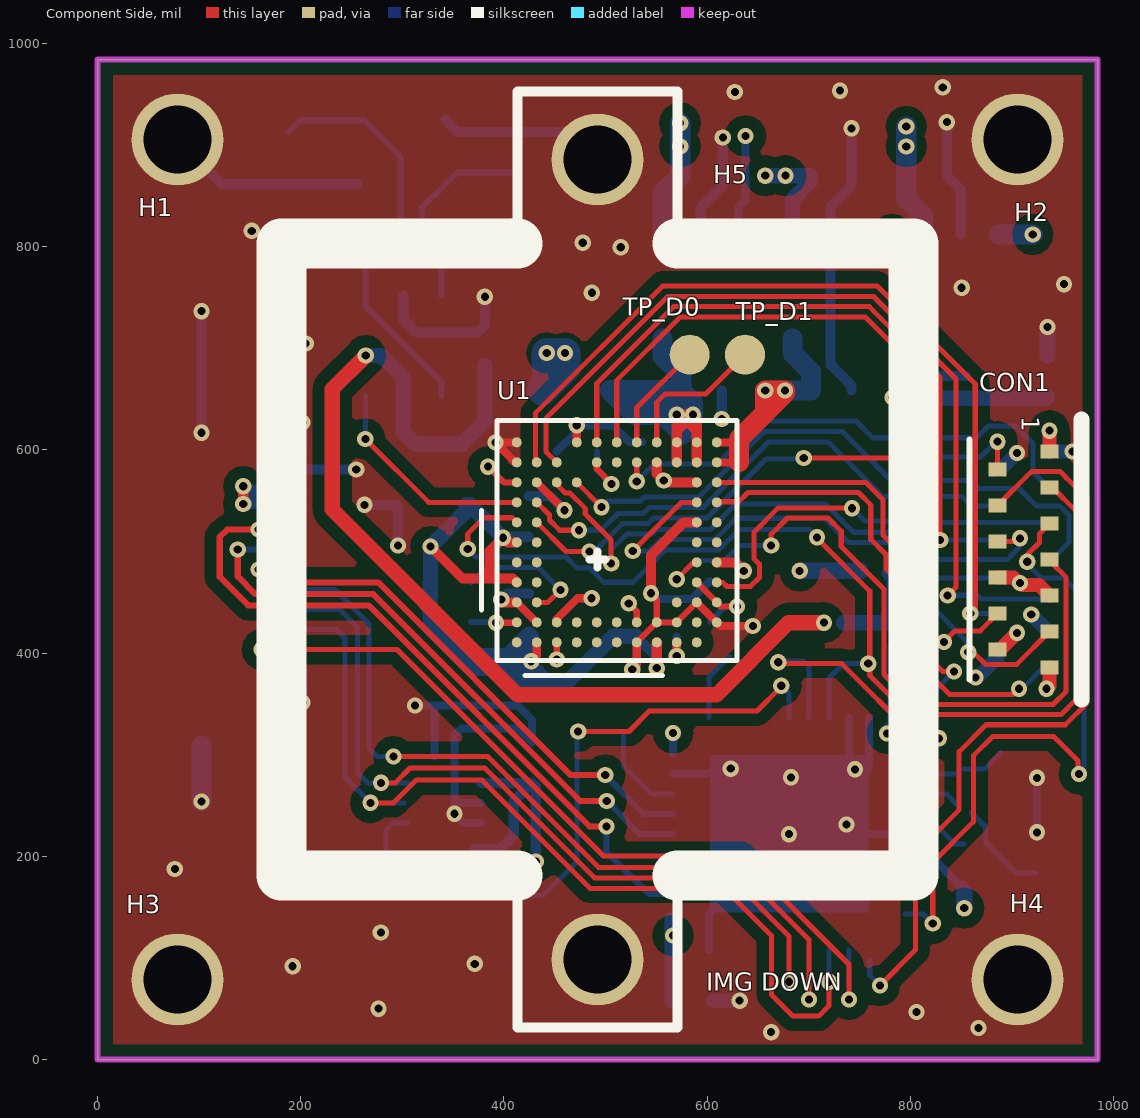
[diagram p0: Component Side view]
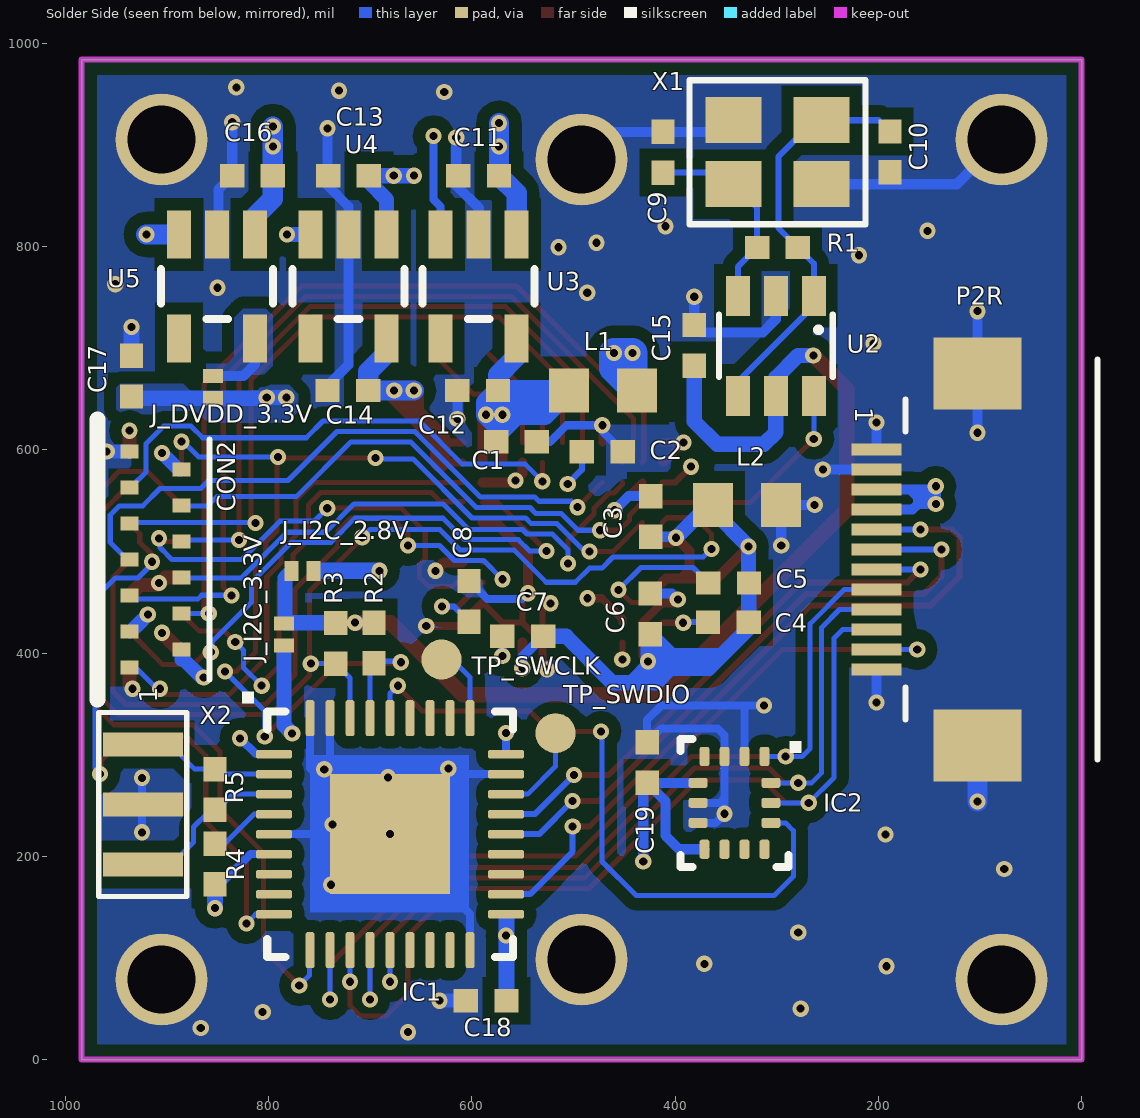
[diagram p1: Solder Side view, seen from below]
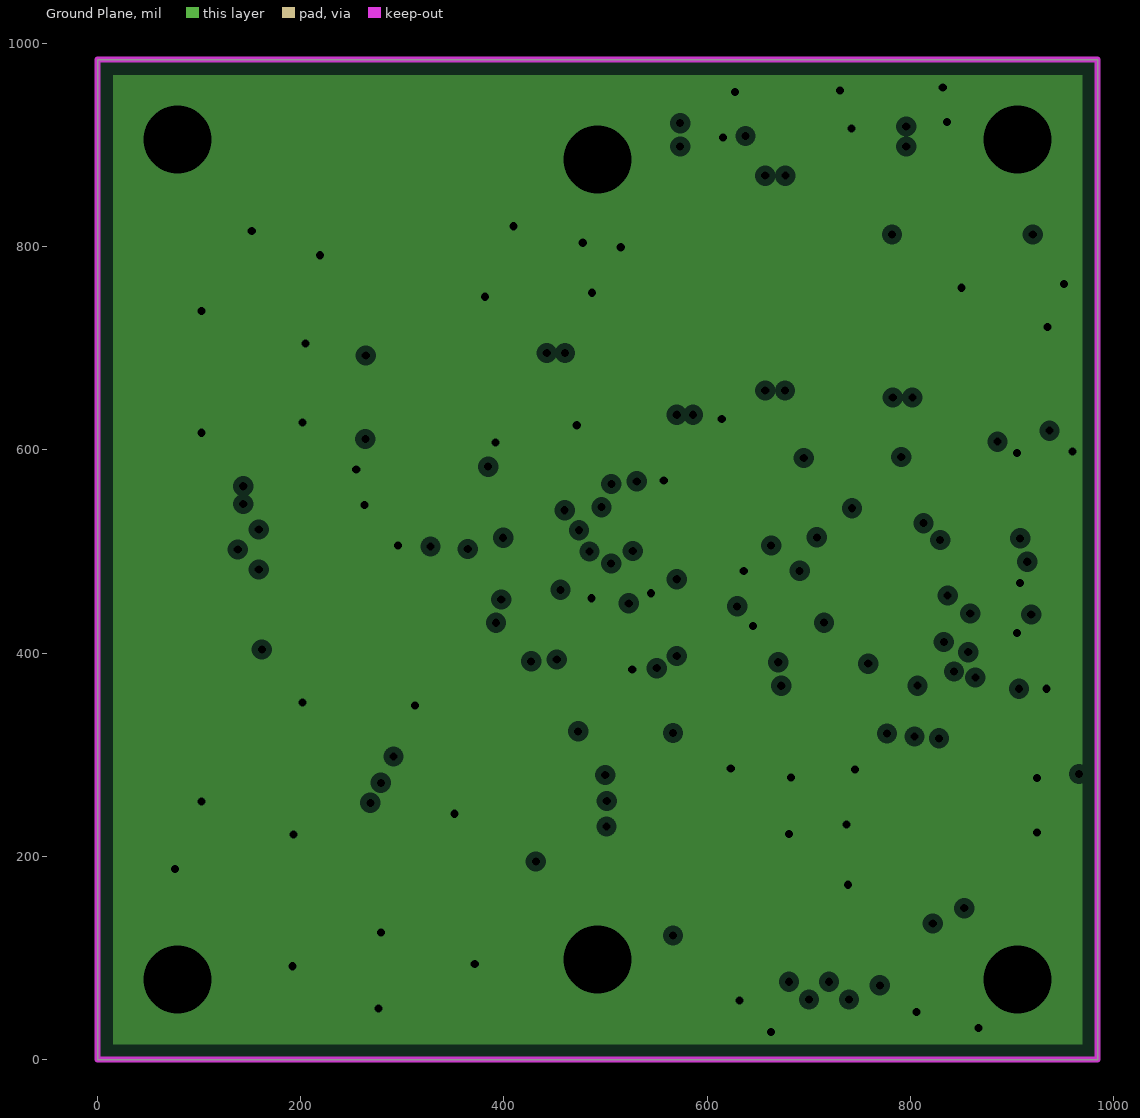
[diagram p2: Ground Plane, clearances drawn from the general rule]
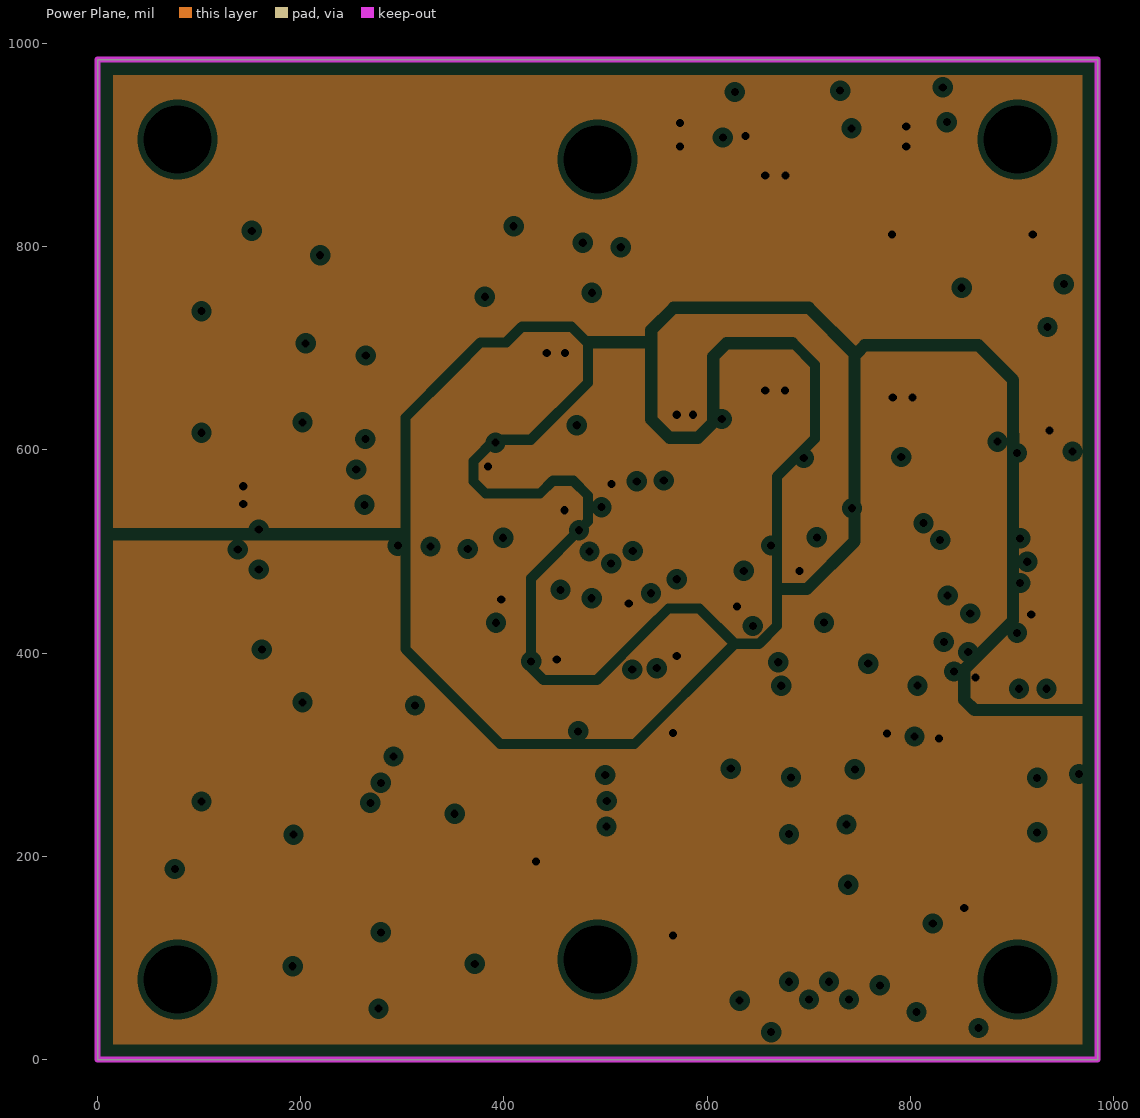
[diagram p3: Power Plane, clearances drawn from the general rule]
# Altium PCB MISC84416.PcbDoc
Units mil, origin at the board's own origin, x right, y up, seen from the top; angles counter-clockwise.
Board outline 984.25 x 984.25 mil, 4 copper layers (Component Side, Ground Plane, Power Plane, Solder Side), stack 33.234 mil thick; 50 components, 46 nets, 258 pads, 152 vias.

## Layer stack, top to bottom
Component Side: signal copper 1.4
Dielectric: core 12.6, FR-4, Dk 4.8
Ground Plane: plane copper 1.4169, net DGND
Dielectric: prepreg 5, Dk 4.2
Power Plane: plane copper 1.4169, net (Multiple Nets)
Dielectric: core 10, Dk 4.2
Solder Side: signal copper 1.4

## Board outline
0,0 984.25,0 984.25,984.25 0,984.25

## Design rules (kind name [scope] priority, off if disabled: settings)
AssemblyTestPointUsage [All] p1 off:
AssemblyTestpoint [All] p1 off: testpointundercomponent=TRUE minsize=40 maxsize=100 preferedsize=60 minholesize=0 maxholesize=40 preferedholesize=32 testpointgrid=1 usegrid=TRUE gridtolerance=0.01 allowsidetop=TRUE allowsidebottom=TRUE
Clearance Clearance_1 [InPolygon] p1: gap=12
Clearance [All] p2: gap=5
ComponentClearance [All] p1 off: gap=10 collisioncheckmode=3 verticalgap=10 showdistances=FALSE
DiffPairsRouting [All] p1 off: maxlimit=10 minlimit=10 mostfreqgap=10 maxuncoupledlength=500
FabricationTestPointUsage [All] p1 off: valid=0 allowmultiple=FALSE
FabricationTestpoint [All] p1 off: side=3 testpointundercomponent=TRUE minsize=40 maxsize=100 preferedsize=60 minholesize=0 maxholesize=40 preferedholesize=32 testpointgrid=1 allowsidetop=TRUE allowsidebottom=TRUE usegrid=TRUE gridtolerance=0.01
FanoutControl Fanout_BGA [IsBGA] p1 off: bgadir=Out bgaviamode=Centered fanoutstyle=Auto fanoutdirection=Alternating viagrid=1 // Fanout_BGA (Default Rule)
FanoutControl Fanout_LCC [IsLCC] p2 off: bgadir=Out bgaviamode=Centered fanoutstyle=Auto fanoutdirection=Alternating viagrid=1 // Fanout_LCC (Default Rule)
FanoutControl Fanout_SOIC [IsSOIC] p3 off: bgadir=Out bgaviamode=Centered fanoutstyle=Auto fanoutdirection=Alternating viagrid=1 // Fanout_SOIC (Default Rule)
FanoutControl Fanout_Small [(CompPinCount < 5)] p4 off: bgadir=Out bgaviamode=Centered fanoutstyle=Auto fanoutdirection=OutThenIn viagrid=1 // Fanout_Small (Default Rule)
FanoutControl Fanout_Default [All] p5 off: bgadir=Out bgaviamode=Centered fanoutstyle=Auto fanoutdirection=Alternating viagrid=1 // Fanout_Default (Default Rule)
Height [All] p1 off: minheight=0 maxheight=1000 prefheight=500
HoleSize [All] p1 off: absolutevalues=TRUE maxlimit=500 minlimit=1 maxpercent=80.000 minpercent=20.000
HoleToHoleClearance [All] p1 off: gap=0 allowstackedmicrovias=TRUE
LayerPairs [All] p1 off: enforce=TRUE
MinimumSolderMaskSliver [All] p1 off: minsoldermaskwidth=0
NetAntennae [All] p1 off: netantennaetolerance=0
PasteMaskExpansion [All] p1 off: expansion=0
PlaneClearance [All] p1: clearance=6
PlaneConnect [All] p1: planeconnectstyle=Direct reliefexpansion=20 reliefentries=4 reliefconductorwidth=10 reliefairgap=10
PolygonConnect [All] p1: connectstyle=Direct reliefconductorwidth=10 reliefentries=4 polygonreliefangle="90 Angle"
RoutingCorners [All] p1 off: cornerstyle=45-Degree minsetback=100 maxsetback=100
RoutingLayers [All] p1 off: top layer_v5=TRUE bottom layer_v5=TRUE
RoutingPriority [All] p1 off: routingpriority=0
RoutingTopology [All] p1 off: topology=Shortest
RoutingVias [All] p1: holewidth=8 width=16 viastyle="Through Hole" minholewidth=8 minwidth=16 maxholewidth=8 maxwidth=16
SilkToSilkClearance [All] p1 off: silktosilkclearance=0
SilkscreenOverComponentPads SilkToSolderMaskClearance [IsPad] p1 off: minsilkscreentomaskgap=0
SolderMaskExpansion [All] p1 off: expansion=4
Width [All] p1: maxlimit=200 minlimit=5 preferedwidth=5
2 further rules are at their usual default settings.

## Components (designator, comment, footprint, x,y, rotation, side; value= is the part's Value field where it differs from the comment)
C1 "1uF" RCL_C0402_TI 556.08,608 r180 bottom
C2 "0.1uF" RCL_C0402_TI 471.75,598.33 r0 bottom
C3 "0.1uF" RCL_C0402_TI 424.2,534.53 r270 bottom
C4 "0.1uF" RCL_C0402_TI 347.7,430.5 r180 bottom
C5 "0.1uF" RCL_C0402_TI 347.27,469.12 r180 bottom
C6 "0.1uF" RCL_C0402_TI 424.51,438.74 r90 bottom
C7 "0.1uF" RCL_C0402_TI 550.02,416.54 r0 bottom
C8 "0.1uF" RCL_C0402_TI 602.85,451.07 r90 bottom
C9 "10pF" RCL_C0402_TI 411.93,893.03 r90 bottom
C10 "10pF" RCL_C0402_TI 188.5,893.43 r270 bottom
C11 "1uF" RCL_C0402_TI 593.39,869.96 r0 bottom
C12 "1uF" RCL_C0402_TI 594.37,658.47 r0 bottom
C13 "1uF" RCL_C0402_TI 721.44,869.96 r0 bottom
C14 "1uF" RCL_C0402_TI 722.18,658.47 r0 bottom
C15 "0.1uF" RCL_C0402_TI 381.18,702.99 r90 bottom
C16 "1uF" RCL_C0402_TI 815.93,869.96 r0 bottom
C17 "1uF" RCL_C0402_TI 935.04,672.66 r90 bottom
C18 "0.1uF" RCL_C0402_TI 586,58 r0 bottom
C19 "0.1uF" RCL_C0402_TI 427.62,292.29 r270 bottom
CON1 "13P-0.5-36AWG" 13P-0.5-36AWG 858.27,492.13 r90 top
CON2 "13P-0.5-36AWG" 13P-0.5-36AWG 858.27,492.13 r270 bottom
H1 "MOUNT-HOLE1.7" MOUNT-HOLE1.7#1 3575.07,942.44 r0 top locked
H2 "MOUNT-HOLE1.7" MOUNT-HOLE1.7#2 3725.07,942.44 r0 top locked
H3 "MOUNT-HOLE1.7" MOUNT-HOLE1.7#3 2556.96,942.44 r0 top locked
H4 "MOUNT-HOLE1.7" MOUNT-HOLE1.7#4 2727.04,942.44 r0 top locked
H5 "MOUNT-LENS" MOUNT-LENS-M12-1.6 492.12,492.11 r90 top locked
IC1 "GD32F103TBU6 36pin QFN" GD32_QFN36 680.61,221.85 r180 bottom locked
IC2 "QMI8658C" LGA14_3X2.5 341.57,252.68 r270 bottom
J_DVDD_3.3V "JUMPER_2P_MIN" JUMPER_2P_MIN 854.72,661.81 r270 bottom
J_I2C_2.8V "JUMPER_2P_MIN" JUMPER_2P_MIN 767,481 r180 bottom
J_I2C_3.3V "JUMPER_2P_MIN" JUMPER_2P_MIN 785.04,418.5 r270 bottom
L1 "470R L" RCL_L0603 471.08,658.63 r0 bottom
L2 "470R L" RCL_L0603 329.07,545.99 r0 bottom
P2R "FPC-12P-0.5-H-NORM" FPC-12P-0.5-H-NORM 177.16,492.11 r90 bottom locked
R1 "1M" RCL_R0402_TI 299.29,799.29 r180 bottom
R2 "2.2K" RCL_R0402_TI 696.42,410 r270 bottom
R3 "2.2K" RCL_R0402_TI 734.13,409.65 r270 bottom
R4 "2.2K" RCL_R0402_TI 852.87,192.36 r270 bottom
R5 "1M" RCL_R0402_TI 852.91,265.87 r270 bottom
TP_D0 "" TP-1#1 582.76,693.74 r270 top
TP_D1 "" TP-1#1 637.24,693.74 r270 top
TP_SWCLK "" TP-1#2 629.92,396.85 r90 bottom
TP_SWDIO "" TP-1#1 517.72,321.26 r90 bottom
U1 "CMOS sensor" BGA71_5.99X5.84 492.12,492.11 r180 top locked
U2 "NL27WZU04DTT" SOT23-6 300.94,702.56 r0 bottom
U3 "ME6219SMD-2.8V" SOT23-5 593.39,760.91 r0 bottom
U4 "ME6219SMD-1.5V" SOT23-5 721.48,760.91 r0 bottom
U5 "ME6211" SOT23-5 850.79,760.91 r0 bottom
X1 "24M/9pF" EPSON-TSX3225 299.17,893.03 r90 bottom
X2 "4MHz" XTAL_4.5X2.0 924,251 r90 bottom

## Footprints (in the part's own frame and the unit in brackets; to place one, negate y for a bottom-side part, rotate by r counter-clockwise, add the part's x,y. Pads: shape width x height; smd on the part's side, far side on the other; paste and mask are expansions set on the pad)
13P-0.5-36AWG [mm]
  rect 0.35x0.45 smd paste+0.13: P$1(2.7,-2) P$2(2.25,-0.7) P$3(1.8,-2) P$4(1.35,-0.7) P$5(0.9,-2) P$6(0.45,-0.7) P$7(0,-2) P$8(-0.45,-0.7) P$9(-0.9,-2) P$10(-1.35,-0.7) P$11(-1.8,-2) P$12(-2.25,-0.7) P$13(-2.7,-2)
  silkscreen extent -3.5,-2.8 3.5,0
BGA71_5.99X5.84 [mm] "BGA71_5.99X5.84"
  round 0.25 smd paste+0.04: A2(-2.48,2.07) A3(-1.98,2.07) A4(-1.48,2.07) A5(-0.98,2.07) A6(-0.48,2.07) A7(0.02,2.07) A8(0.52,2.07) A9(1.02,2.07) A10(1.52,2.07) A11(2.02,2.07) B1(-2.98,1.57) B2(-2.48,1.57) B3(-1.98,1.57) B4(-1.48,1.57) B5(-0.98,1.57) B6(-0.48,1.57) B7(0.02,1.57) B8(0.52,1.57) B9(1.02,1.57) B10(1.52,1.57) B11(2.02,1.57) C1(-2.98,1.07) C2(-2.48,1.07) C3(-1.98,1.07) C10(1.52,1.07) C11(2.02,1.07) D1(-2.98,0.57) D2(-2.48,0.57) D10(1.52,0.57) D11(2.02,0.57) E1(-2.98,0.07) E2(-2.48,0.07) E10(1.52,0.07) E11(2.02,0.07) F1(-2.98,-0.43) F2(-2.48,-0.43) F10(1.52,-0.43) F11(2.02,-0.43) G1(-2.98,-0.93) G2(-2.48,-0.93) G10(1.52,-0.93) G11(2.02,-0.93) H1(-2.98,-1.43) H2(-2.48,-1.43) H10(1.52,-1.43) H11(2.02,-1.43) I1(-2.98,-1.93) I2(-2.48,-1.93) I8(0.52,-1.93) I9(1.02,-1.93) I10(1.52,-1.93) I11(2.02,-1.93) J1(-2.98,-2.43) J2(-2.48,-2.43) J3(-1.98,-2.43) J4(-1.48,-2.43) J5(-0.98,-2.43) J6(-0.48,-2.43) J7(0.02,-2.43) J9(1.02,-2.43) J10(1.52,-2.43) J11(2.02,-2.43) K2(-2.48,-2.93) K3(-1.98,-2.93) K4(-1.48,-2.93) K5(-0.98,-2.93) K6(-0.48,-2.93) K7(0.02,-2.93) K8(0.52,-2.93) K11(2.02,-2.93)
  round 0.25 smd paste+0.04 mask+0.102: K1(-2.98,-2.93)
  silkscreen extent -3.48,-3.48 2.9,2.9
EPSON-TSX3225 [mm] "EPSON-TSX3225"
  rect 1.15x1.4 smd paste+0: 1(-0.8,1.1) 2(-0.8,-1.1) 3(0.8,-1.1) 4(0.8,1.1)
  silkscreen extent -1.8,-2.2 1.8,2.2
FPC-12P-0.5-H-NORM [mm]
  rect 1.8x2.2 smd: M(-4.65,-1.9) M(4.65,-1.9)
  rect 0.3x1.25 smd paste-0.75: P$1(2.75,0.625) P$2(2.25,0.625) P$3(1.75,0.625) P$4(1.25,0.625) P$5(0.75,0.625) P$6(0.25,0.625) P$7(-0.25,0.625) P$8(-0.75,0.625) P$9(-1.25,0.625) P$10(-1.75,0.625) P$11(-2.25,0.625) P$12(-2.75,0.625)
  silkscreen extent -5,-4.9 5,-0.1
GD32_QFN36 [mm]
  rrect50% 0.9x0.22 smd paste-0.9: 1(-2.9,2) 2(-2.9,1.5) 3(-2.9,1) 4(-2.9,0.5) 5(-2.9,0) 6(-2.9,-0.5) 7(-2.9,-1) 8(-2.9,-1.5) 9(-2.9,-2) 19(2.9,-2) 20(2.9,-1.5) 21(2.9,-1) 22(2.9,-0.5) 23(2.9,0) 24(2.9,0.5) 25(2.9,1) 26(2.9,1.5) 27(2.9,2)
  rect 3x3 smd paste-3: 5(0,0)
  rrect50% 0.22x0.9 smd paste-0.9: 10(-2,-2.9) 11(-1.5,-2.9) 12(-1,-2.9) 13(-0.5,-2.9) 14(0,-2.9) 15(0.5,-2.9) 16(1,-2.9) 17(1.5,-2.9) 18(2,-2.9) 28(2,2.9) 29(1.5,2.9) 30(1,2.9) 31(0.5,2.9) 32(0,2.9) 33(-0.5,2.9) 34(-1,2.9) 35(-1.5,2.9) 36(-2,2.9)
  silkscreen extent -3.7,-3.07 3.07,3.56
JUMPER_2P_MIN [mm]
  rect 0.35x0.5 smd paste-0.05: 1(-0.275,0) 2(0.275,0)
LGA14_3X2.5 [mm]
  rrect50% 0.48x0.25 smd paste-0.48: 1(-1.16,0.75) 2(-1.16,0.25) 3(-1.16,-0.25) 4(-1.16,-0.75) 8(1.16,-0.75) 9(1.16,-0.25) 10(1.16,0.25) 11(1.16,0.75)
  rrect50% 0.25x0.48 smd paste-0.48: 5(-0.5,-0.91) 6(0,-0.91) 7(0.5,-0.91) 12(0.5,0.91) 13(0,0.91) 14(-0.5,0.91)
  silkscreen extent -1.6,-1.35 1.6,1.68
MOUNT-HOLE1.7#1 [mm]
  round 2.3 hole 1.7: MOUNT(-88.807,-0.938)
MOUNT-HOLE1.7#2 [mm]
  round 2.3 hole 1.7: MOUNT(-71.617,-0.938)
MOUNT-HOLE1.7#3 [mm]
  round 2.3 hole 1.7: MOUNT(-62.947,-21.938)
MOUNT-HOLE1.7#4 [mm]
  round 2.3 hole 1.7: MOUNT(-46.267,-21.938)
MOUNT-LENS-M12-1.6 [mm]
  round 2.3 hole 1.7: MOUNT(-10,0) MOUNT(10,0)
  silkscreen extent -11.7,-7.9 11.7,7.9
RCL_C0402_TI [mil]
  rect 24x23 smd: 1(-20,0) 2(20,0)
RCL_L0603 [mm]
  rect 1x1.1 smd: 1(-0.85,0) 2(0.85,0)
RCL_R0402_TI [mil]
  rect 24x23 smd: 1(-20,0) 2(20,0)
SOT23-5 [mm]
  rect 0.6x1.2 smd: 1(-0.95,-1.3) 2(0,-1.3) 3(0.95,-1.3) 4(0.95,1.3) 5(-0.95,1.3)
  silkscreen extent -1.4,-0.43 1.4,0.81
SOT23-6 [mm]
  rect 0.6x1 smd: 1(-0.95,-1.25) 2(0,-1.25) 3(0.95,-1.25) 4(0.95,1.25) 5(0,1.25) 6(-0.95,1.25)
  silkscreen extent -1.42,-0.78 1.42,0.78
TP-1#1 [mm]
  round 1 smd paste-1: 1(0,0)
TP-1#2 [mm]
  round 1 smd paste-1: 1(-0.08,0)
XTAL_4.5X2.0 [mm] "XTAL_4.5X2.0"
  rect 0.6x2 smd paste-0.15: 1(-1.5,0) 2(0,0) 3(1.5,0)
  silkscreen extent -2.3,-1.1 2.3,1.1

## Part data
C1 C2 C3 C4 C5 C6 C7 C8 C9 C10 C11 C12 C13 C14 C15 C16 C17 C18 C19: library part RCL_C-EUC0402_TI
IC1: library part GD32F103TBU6
L1 L2: library part RCL_L-USL0603
R1 R2 R3 R4 R5: library part RCL_R-EUR0402_TI
TP_D0 TP_D1 TP_SWCLK TP_SWDIO: library part TP-1
U1: library part OV5640, "1/4INCH"
U3 U4: library part ME6219SMD
U5: library part ME6211SMD
X1: library part XTAL_EPSON_3225
X2: library part XTAL_MURATA-4.5X2.0

## Via types
v1: diameter 16, hole 8, Component Side to Solder Side, tented both sides, 117 vias
v2: diameter 16, hole 8, Component Side to Solder Side, 35 vias

## Nets (pads, with @x,y where several pads share a name; then routed paths per layer and width w, separated by ;. In a path a pad name is that pad's centre, name@x,y a point inside that pad or via, vN(x,y) a via of type N, cw(c..) or ccw(c..) an arc to the next point about the centre after c; other vN are vias at no path point)
AGND: C3.2 C4.2 C5.2 C6.1 C7.1 L2.2 U1.A4 U1.A10 U1.D11 U1.F11 | length 1036.7
  Component Side w8: v1(426.75,391.97) 432.28,397.5 U1.A10
  Component Side w10: v1(327.7,504.97) 359.16,473.51 376.28,473.51 ; U1.D11 408.75,473.51 394.31,473.51 ; U1.F11 403.7,509.04 v1(399.15,513.59) 385.81,500.24 385.81,483.04 ; v1(550.39,385.25) U1.A4 ; 376.28,473.51 385.81,483.04 ; 376.28,473.51 385.81,473.51 ; 385.81,473.51 385.81,482.01 ; 385.81,473.51 394.31,473.51 ; 385.81,482.01 394.31,473.51 ; 385.81,482.01 385.81,483.04
  Solder Side w8: C6.1 424.51,394.22 v1(426.75,391.97)
  Solder Side w10: v1(399.15,513.59) 400.09,514.53 C3.2 ; 404.51,385.12 411.36,391.97 412.78,393.39 417.03,397.64 420.49,401.1 423.7,401.1 ; C7.1 550.39,396.17 v1(550.39,385.25)
  Solder Side w15: C5.2 327.27,424.57 354.19,397.64 ; C4.2 v1(327.7,504.97) 362.54,539.81 L2.2 366.75,545.99 v1(399.15,513.59) ; 411.36,391.97 414.19,391.97 ; C7.1 507.22,416.54 461.48,370.79 443.21,370.79 ; 354.19,397.64 366.71,385.12 404.51,385.12 418.84,370.79 428.33,370.79 ; 354.19,397.64 403.41,397.64 ; 403.41,397.64 C6.1 426.75,416.5 v1(426.75,391.97) v1@423.7,391.97 ; 403.41,397.64 408.52,397.64 ; 408.52,397.64 412.78,393.39 414.19,391.97 ; 408.52,397.64 417.03,397.64 420.24,397.64 423.7,401.1 v1@423.7,391.97 ; 414.19,391.97 v1@423.7,391.97 ; 414.19,391.97 428.33,377.84 428.33,370.79 ; v1@423.7,391.97 423.7,390.3 443.21,370.79 ; 428.33,370.79 443.21,370.79
AVDD_2.8V: C3.1 C6.2 C7.2 L1.1 U1.A3 U1.B10 U1.C11 U1.I10 | length 283.1
  Component Side w8: U1.C11 U1.B10 ; U1.I10 v1(459.7,540.67) ; v1(570.07,397.26) U1.A3
  Component Side w10: v1(397.34,452.8) 400.16,449.98 U1.C11
  Solder Side w8: C7.2 570.07,416.49 v1(570.07,397.26)
  Solder Side w10: v1(397.34,452.8) 403.29,458.74 C6.2 ; C3.1 445.84,554.53 v1(459.7,540.67)
  Solder Side w30: L1.1 L1.1@442.07,663.07 ; L1.1@442.07,663.07 v1(442.07,695.44) v1(460.1,695.44) 460.1,681.11 L1.1@442.07,663.07
CAM_SCL: CON1.P$2 IC1.33 R2.2 U1.G10 | length 1091.8
  Component Side w5: U1.G10 460.96,500.04 v1(484.23,500.04) ; v2(670,391) v2@675,391 ; v2@675,390 732,390 v2(804,318) ; v2(695,592) v2@792,592 ; v2@792,593 v2@792,592 ; v2@844,382 v2(843,382) 832,382 813,401 813,487 803,497 803,509 792,520 v2@792,592 ; CON1.P$2 v2(885.83,608.17)
  Solder Side w5: v1(484.23,500.04) 489,500.04 516.4,527.44 541.63,527.44 547.18,533 599.86,533 657.87,591 691,591 v2@693,593 ; v2(670,391) 671,392 R2.2@695,392 ; IC1.33 R2.2@700.3,386.12 ; v2@794,593 869,593 v2@882,606 ; v2(804,318) 804,343 v2(843,382) ; v2@882,608.17 v2(885.83,608.17)
  other v2: 791,593
CAM_SDA: CON1.P$3 IC1.34 R3.2 U1.G11 | length 1139.3
  Component Side w5: v1(364.35,502.48) 364.35,517.44 380.22,533.31 408,533.31 U1.G11 ; v2@709,512 760,461 760,378 798.5,339.5 903,339.5 948.36,339.5 963.37,354.51 963.37,539.63 940.01,562.99 CON1.P$3
  Solder Side w5: v1(364.35,502.48) 372.22,494.61 461.08,494.61 472.07,483.63 484.35,483.63 498.21,469.77 526.91,469.77 558.88,501.74 611.67,501.74 631.59,521.66 700.34,521.66 v2(708,514) ; IC1.34 719.98,375.49 R3.2 v1(758.57,389.65)
CLK: IC1.12 IC2.13 P2R.P$10 | length 900.5
  Component Side w5: v1(268.53,252.68) 291.35,252.68 313.72,275.04 378.22,275.04 484.8,168.47 616.75,168.47 663.17,122.05 663.17,64.02 684.51,42.68 709.78,42.68 719.98,52.88 v1(719.98,76.62)
  Solder Side w5: P2R.P$10 235.08,423.21 243.48,414.81 243.48,277.72 v1(268.53,252.68) IC2.13@301.36,252.68 ; v1(719.98,76.62) IC1.12
CS_IMU: IC1.32 IC2.12 | length 663.7
  Component Side w5: v1@472,321 v1@474,323 ; v1@473.92,323 v1(473,323) v1@474,323 ; v1@672,366 649,343 543,343 523,323 v1@474,323 ; v1@672,367.92 v1(672.97,367.92)
  Solder Side w5: IC2.12 291.47,232.99 283.72,225.24 283.72,180.24 302.54,161.42 438.41,161.42 472,195.02 v1@472,321 ; v1(473,323) v1@473.92,323 ; v1(672.97,367.92) 680.61,360.28 IC1.32
CS_LASER: IC1.11 P2R.P$11 | length 829.3
  Component Side w5: v1(161.69,403.53) 294.72,403.53 497.97,200.28 632.93,200.28 739.67,93.55 v1(739.67,59.18)
  Solder Side w5: v1(161.69,403.53) P2R.P$11 ; v1(739.67,59.18) IC1.11
D0: TP_D0.1 U1.K5 | length 107.8
  Component Side w5: U1.K5 530.7,641.69 TP_D0.1
D1: TP_D1.1 U1.K4 | length 145.7
  Component Side w5: U1.K4 550.39,646.87 558.8,655.28 598.78,655.28 TP_D1.1
D2: CON2.P$11 U1.J5 | length 500.3
  Component Side w5: v1(530.7,569.09) U1.J5
  Solder Side w5: v1(530.7,569.09) 547.64,586.03 609.59,586.03 651.99,628.43 746.57,628.43 763,612 865,612 876.67,623.67 903.33,623.67 920.65,606.35 920.65,578.35 CON2.P$11@935,564
D3: CON2.P$10 U1.H10 | length 528.9
  Component Side w5: U1.H10 444.78,535.91 444.78,531.11 454.94,520.95 v1(473.92,520.95)
  Solder Side w5: v1(473.92,520.95) 495.53,520.95 512.15,537.56 537.11,537.56 542.89,543.35 595.85,543.35 660.26,607.76 719.24,607.76 773,554 851,554 860,545 CON2.P$10@885,545
D4: CON2.P$9 U1.K6 | length 682.3
  Component Side w5: U1.K6 511.02,668.56 573.17,730.71 755.77,730.71 817.47,669.02 817.47,530.47 815,528 v2(813,528)
  Solder Side w5: v2(813,528) 813.5,528.5 931.5,528.5 CON2.P$9@932,528
D5: CON2.P$8 U1.K7 | length 672.5
  Component Side w5: U1.K7 491.33,665.49 566.87,741.03 759.6,741.03 829.32,671.31 v2(829.32,511.32)
  Solder Side w5: v2(829.32,511.32) CON2.P$8@885.68,511.32
D6: CON2.P$7 U1.I8 | length 606.1
  Component Side w5: U1.I8 v1(496.04,543.7)
  Solder Side w5: v1(496.04,543.7) 501.84,549.49 534.11,549.49 538.29,553.67 591.79,553.67 656.28,618.15 732.85,618.15 781,570 859,570 867,562 907,562 924,545 947,545 956,536 956,509 CON2.P$7@942,495
D7: CON2.P$6 U1.I9 | length 548.7
  Component Side w5: U1.I9 451.96,565.98 460.22,557.72 464.78,557.72 479.98,542.52 479.98,536.89 505.47,511.4 v1(505.47,488.27)
  Solder Side w5: v1(505.47,488.27) 505.47,501.79 520.93,517.25 545.81,517.25 550.33,521.78 603.17,521.78 628.39,547 716,547 744,519 782,519 827,474 CON2.P$6@882,474 ; CON2.P$6@882,474.41 CON2.P$6 ; CON2.P$6@885.83,474 CON2.P$6@887,474
D8: CON2.P$5 U1.J9 | length 852.8
  Component Side w5: U1.J9 441.2,598.54 441.2,631.03 561.28,751.11 763.67,751.11 844.82,669.95 844.82,464.82 v2@837,457
  Solder Side w5: v2(836.69,456.69) v2@840,456.69 ; v2@840,457 866,457 869.5,453.5 936.5,453.5 CON2.P$5@937,453
D9: CON2.P$4 U1.J10 | length 825.8
  Component Side w5: U1.J10 430.89,589.17 430.89,636.15 556.2,761.46 767.45,761.46 863.88,665.04 863.88,443.88 v2(859,439)
  Solder Side w5: v2(859,439) CON2.P$4@883,439
DGND: C1.2 C2.1 C8.2 C9.2 C10.2 C11.2 C12.2 C13.2 C14.2 C15.2 C16.2 C17.2 C18.2 C19.1 CON1.P$8 CON1.P$9 CON1.P$12 CON1.P$13 CON2.P$12 CON2.P$13 H1.MOUNT H2.MOUNT H3.MOUNT H4.MOUNT H5.MOUNT IC1.5 IC1.18 IC1.26 IC1.35 IC1.36 IC2.2 IC2.3 IC2.6 IC2.7 L2.1 P2R.M P2R.P$1 P2R.P$2 P2R.P$12 U1.A5 U1.B1 U1.B3 U1.B4 U1.B9 U1.C2 U1.E1 U1.G2 U1.I2 U1.J4 U1.J11 U1.K8 U1.K11 U2.2 U3.2 U4.2 U5.2 X1.2 X1.4 X2.2 | length 3349.1
  Component Side w6: U1.A5 U1.B4 ; v1(544.74,459.02) 550.39,453.38 U1.B4 ; U1.C2 U1.B3 U1.B4
  Component Side w8: U1.J11 411.14,587.78 v1(391.67,607.25) 412.37,607.25 U1.K11 ; U1.B9 451.96,433.76 472.22,454.02 v1(486.32,454.02) ; U1.K8 v1(471.65,624.28) ; v1(526.24,383.98) 530.7,388.44 U1.A5 ; U1.C2 U1.B1 613.08,426.66 v1(644.94,426.66)
  Component Side w10: v1(544.74,459.02) 544.74,496.46 577.01,528.72 U1.G2 ; U1.J4 550.39,576.84 v1(557.22,570) 559.13,568.09 U1.I2 ; U1.E1 616,489.35 ; v2(636,481) 635,482 627.65,489.35 ; 616,489.35 627.65,489.35 ; 616,489.35 627.65,489.35
  Component Side w14: CON1.P$12 888.54,403.54 v2(905,420) ; CON1.P$8 901.59,474.41 907,469 v2(908,469) 910,467 926.7,467 CON1.P$9 ; v2(934,365) 937.01,368.01 CON1.P$13
  Solder Side w8: v1(312.46,348.55) 328.96,348.55 ; IC2.2 331.73,345.77 328.96,348.55 ; IC2.7 360.34,232.99 v1(351.42,241.91) 351.42,257.27 ; IC2.6 356.01,252.68 351.42,257.27 ; C2.1 471.65,618.23 v1(471.65,624.28) 507.08,624.28 523.37,608 C1.2 ; v1(544.74,459.02) 550.57,453.19 584.98,453.19 C8.2 ; IC1.26 621.55,280.91 v1(680.61,221.85) ; IC1.18 601.87,143.11 v1(680.61,221.85) ; IC1.35 739.67,267.09 ; IC1.36 759.35,286.78 739.67,267.09 ; IC1.5@794.78,221.85 IC1.5@694.43,221.85 ; v1(924.73,223.63) 924.73,250.55 v1(924.73,277.25) ; 328.96,348.55 413.56,348.55 427.62,334.49 C19.1 414.11,325.79 358.05,325.79 351.42,319.16 IC2.3 351.42,257.27 ; v1(680.61,221.85) IC1.5@694.43,221.85 ; IC1.5@694.43,221.85 739.67,267.09
  Solder Side w10: H1.MOUNT 122.69,861.54 X1.2 ; v1(102.35,617) 102.35,675.18 v1(102.35,736.63) ; v1(201.76,351.53) P2R.P$12 ; P2R.P$2 v1(254.65,580.69) ; P2R.P$1 v1(201.76,627.14) ; v1(262.7,545.99) L2.1 v1(295.61,505.87) ; U2.2 300.94,728.53 313.8,715.67 373.86,715.67 C15.2 v1(381.18,750.81) ; X1.4 353.98,913.03 C9.2 464.9,913.03 H5.MOUNT@492.12,885.81 ; U3.2 593.39,838.25 615.41,860.28 v1(615.41,907.48) ; v1(614.37,630.53) C12.2 ; v1(742.07,916.54) 742.07,860.24 721.48,839.65 U4.2 721.48,683.78 742.18,663.07 C14.2 ; v1(835.93,922.64) C16.2 849.57,856.32 U5.2@849.57,812.09
  Solder Side w14: C18.2 v1(632,58) ; CON2.P$12 888.71,580.71 v2(905,597) ; v2@904,420 v2(905,420) ; CON2.P$13 v2(959.57,598.43)
  Solder Side w16: C17.2 v1(935,721)
  Solder Side w20: v1(102.35,254.05) P2R.M@102.35,309.04
  other v1: 663,27 867,31 806,46.78 276.48,50.08 191.99,91.85 371.28,94.22 278.84,125.16 738.76,172.09 76.04,187.6 192.93,221.42 737.15,231.42 682.58,277.76 745.41,285.67 623.25,286.3 204.82,704.89 486.52,754.77 850.45,759.61 951.12,763.19 219.07,791.7 514.9,799.53 477.54,803.98 151.71,815.63 409.55,820.2 627.22,952.33 730.85,953.63 831.91,956.89
DOVDD_2.8V: C1.1 C12.1 J_I2C_2.8V.2 L1.2 U1.J2 U1.J3 U1.K2 U1.K3 U3.5 | length 704.4
  Component Side w10: U1.J3 U1.K3 570.07,618.7 ; U1.J2 U1.K2 589.76,618.65 ; 570.07,618.7 v1(570.07,634.7) v1@578.37,634.7 ; 570.07,618.7 579.89,628.52 ; v1@578.37,634.7 v1(586.07,634.7) ; v1@578.37,634.7 v1@582.22,630.85 ; 579.89,628.52 v1@582.22,630.85 ; 579.89,628.52 589.76,618.65 ; v1@582.22,630.85 v1(586.07,634.7) ; v1(586.07,634.7) 589.76,631.02 589.76,618.65
  Solder Side w10: v1(570.07,634.7) v1@570.37,635
  Solder Side w16: v2(691,481) J_I2C_2.8V.2@751,481
  Solder Side w20: U3.5 555.98,692.11 574.37,673.72 C12.1 ; L1.2@504.7,658.47 L1.2 574.21,658.63 C12.1 ; L1.2@504.7,658.47 L1.2@515.12,648.05 ; L1.2@504.7,658.47 525.53,658.47 ; L1.2@515.12,648.05 L1.2@515.65,647.52 ; L1.2@515.12,648.05 525.53,658.47 ; L1.2@515.65,647.52 563.43,647.52 C12.1 ; L1.2@515.65,647.52 528.47,634.7 556.4,634.7 ; 525.53,658.47 C12.1 ; 556.4,634.7 v1(570.07,634.7) v1@574.37,634.7 ; 556.4,634.7 C1.1@574.37,616.73 ; C1.1@574.37,616.73 574.37,623 ; C1.1@574.37,616.73 575.59,615.51 575.59,624.22 ; 574.37,623 v1@574.37,634.7 ; 574.37,623 575.59,624.22 ; v1@574.37,634.7 v1(586.07,634.7) ; v1@574.37,634.7 C12.1 ; C12.1 586.07,646.77 v1(586.07,634.7) ; 575.59,624.22 v1(586.07,634.7)
DVDD_1.5V: C2.2 C8.1 C14.1 U1.A9 U1.B5 U1.C1 U1.D2 U1.I11 U1.J1 U1.J7 U1.K1 U4.5 | length 501.6
  Component Side w6: v1(384.39,583.55) 399.84,568.09 U1.I11 ; v1(451.96,393.77) U1.A9 ; U1.J7 491.33,581.37 v1@507.22,565.48 ; v1(522.81,449.02) 530.7,441.13 U1.B5 ; U1.D2 U1.C1 613.4,446.03 v1(629.47,446.03)
  Component Side w8: U1.J1 630.91,587.78 631.36,588.23 ; U1.K1 627.99,607.46 631.36,610.83
  Component Side w20: 631.36,588.23 631.36,610.83 657.18,636.66 ; 657.18,636.66 v1(657.18,658.47) v1(676.59,658.47) 676.59,656.07 657.18,636.66
  Solder Side w6: C2.2 491.75,580.48 v1(505.69,566.54) ; C8.1 617.81,446.03 v1(629.47,446.03)
  Solder Side w20: v1(657.18,658.47) v1(676.59,658.47) C14.1 702.18,677.09 684.07,695.2 U4.5
DVDD_3.3V: C17.1 C18.1 C19.2 IC1.1 IC1.6 IC1.19 IC1.27 IC2.5 IC2.8 J_DVDD_3.3V.2 J_I2C_3.3V.2 R4.2 | length 797
  Solder Side w8: C18.1@566.44,61.44 566.44,136 ; v1(566.44,122.05) 566.44,136 ; IC1.19 566.44,136 ; IC1.27 v1(566.44,321.38) ; IC1.6 818.05,202.17 847.86,172.36 R4.2 ; IC1.1 812.66,300.59 v1(828.25,316.18)
  Solder Side w10: IC2.8 396.16,207.01 409.59,220.44 409.59,254.26 C19.2 ; IC2.5 427.54,272.36 C19.2 ; v1(431.36,194.89) 431.36,268.55 C19.2
  Solder Side w15: v2(777,321) 785.04,329.04 J_I2C_3.3V.2@785.04,406 ; v1(782.68,651.57) v1(801.97,651.57) 802.54,651 J_DVDD_3.3V.2 933.36,650.98 C17.1
  Solder Side w16: C18.1 566,138 ; v1(853,149) R4.2@853,165
EN_STOP1: IC1.20 P2R.P$5 | length 713.7
  Component Side w6: v1(158.6,521.64) 127.56,521.64 120.3,514.37 120.3,475 148.33,446.97 266.71,446.97 484.31,229.37 v1(500.89,229.37)
  Solder Side w6: v1(158.6,521.64) P2R.P$5 ; v1(500.89,229.37) 500.89,204.73 542.81,162.8 IC1.20
GPIO: CON1.P$6 U1.D1 | length 426.1
  Component Side w5: U1.D1@610,469.67 U1.D1 615.33,469.67 619.5,465.5 642.42,465.5 651.5,474.58 651.5,487.5 646,493 646,519 670,543 742.89,543 v2(742.49,542.59) ; CON1.P$6 899,509.84 v2@908,509.84
  Solder Side w5: v2@741,544 741.08,544 v2(742.49,542.59) ; v2@742.45,542.55 755,530 788.73,530 826.73,492 895.32,492 899.5,496.18 899.5,496.42 907,503.92 v2@907,513
  other v2: 908,513
HREF: CON1.P$11 U1.H2 | length 590.1
  Component Side w5: v1(526.71,500.48) 574.65,548.41 U1.H2 ; v2@861,401 862.02,401 873.97,389.04 904.79,389.04 CON1.P$11
  Solder Side w5: v1(526.71,500.48) 543.21,500.48 554.47,511.74 607.42,511.74 628.44,532.76 715.24,532.76 739,509 777.17,509 ; 777.93,508.93 817,469.86 817,450 856,411 v2@856,402
  other v2: 857,401
INTN: IC1.23 P2R.P$6 | length 623.7
  Component Side w6: v1(137.95,501.95) 137.95,475.61 155.37,458.19 271.36,458.19 475.06,254.49 v1(501.16,254.49)
  Solder Side w6: v1(137.95,501.95) P2R.P$6 ; v1(501.16,254.49) 533.8,221.85 IC1.23
MCU_RX: CON1.P$5 IC1.9 | length 631.9
  Component Side w5: v2(822,134) 822,194 862,234 862,299 881,318 941,318 965,294 v2@965,283 ; v2@916,492 916,498 927,509 927,517.55 CON1.P$5 ; v2(966,281) v2@966,283
  Solder Side w5: IC1.9 812.89,143.11 v2(822,134) ; v2@915,487.78 928.78,474 951,474 971,454 971,287 v2@968,284
  other v2: 915,490
MCU_TX: CON1.P$4 IC1.10 | length 751.7
  Component Side w5: v2(770,73) 805,108 805,203 848,246 848,303 874.5,329.5 952.5,329.5 973.75,350.75 973.75,552.25 953.37,572.63 953.37,572.99 947.35,579 919.55,579 CON1.P$4
  Solder Side w5: IC1.10@760,98 760,83 v2(770,73)
MISO: IC1.13 IC2.1 P2R.P$8 | length 841.3
  Component Side w5: v1(291.24,298.35) 384.04,298.35 493.32,189.06 629.23,189.06 700.3,118 v1(700.3,59.18)
  Solder Side w5: P2R.P$8 233.62,462.58 267.15,429.06 267.15,306.22 275.02,298.35 v1(291.24,298.35) IC2.1 ; v1(700.3,59.18) IC1.13
MOSI: IC1.14 IC2.14 P2R.P$9 | length 810.7
  Component Side w5: v1(278.88,272.36) 292.97,272.36 307.58,286.97 380.99,286.97 489.1,178.86 623.13,178.86 680.61,121.38 v1(680.61,76.62)
  Solder Side w5: P2R.P$9 238.27,442.9 255.81,425.36 255.81,282.17 265.61,272.36 v1(278.88,272.36) IC2.14 ; v1(680.61,76.62) IC1.14
NetC4_1: C4.1 U1.B11 | length 45.3
  Component Side w6: v1(392.11,429.92) 412.22,429.92 U1.B11
  Solder Side w6: C4.1 391.54,430.5 v1(392.11,429.92)
NetC5_1: C5.1 U1.C10 | length 132.3
  Component Side w5: U1.C10 443.39,449.98 v1(455.69,462.29)
  Solder Side w5: C5.1 382.44,484.3 433.68,484.3 v1(455.69,462.29)
NetC9_1: C9.1 R1.1 U2.3 X1.1 | length 201.5
  Solder Side w6: U2.3 338.35,780.24 R1.1 319.29,838.35 X1.1 353.98,873.03 C9.1
NetC10_1: C10.1 R1.2 U2.1 U2.4 X1.3 | length 410.1
  Solder Side w6: C10.1 199.61,924.53 X1.3 262.46,924.53 298.44,888.55 298.44,818.44 R1.2 263.54,783.54 U2.1 263.54,741.79 338.35,666.99 U2.4
NetIC1_2: IC1.2 R5.1 X2.3 | length 95.9
  Solder Side w5: IC1.2 R5.1@847.96,280.91 ; R5.1 872.87,285.87 X2.3@889,302
NetIC1_3: IC1.3 R5.2 X2.1 | length 152.5
  Solder Side w5: IC1.3 835.78,261.22 R5.2@846,251 ; R5.2@860.09,242.91 874,229 874,214 904.5,183.5 X2.1@923.73,183.5
NetIC1_4: IC1.4 R4.1 | length 70.2
  Solder Side w5: IC1.4 814.43,241.54 843.61,212.36 R4.1
NetJ_DVDD_3.3V_1: J_DVDD_3.3V.1 U5.5 | length 71.6
  Solder Side w10: U5.5 813.39,684.25 825,672.64 J_DVDD_3.3V.1
PCLK: CON2.P$1 U1.I1 | length 502.3
  Component Side w5: U1.I1 755.91,568.09 773,551 773,516 788,501 788,489 802,475 802,396 831,367 833,365 838.5,359.5 901.5,359.5 v2(907,365) 908,365 v2@910,367
  Solder Side w5: v2@910,365 930.83,385.83 CON2.P$1 ; CON2.P$1@938,383 CON2.P$1@940,385
RESET: CON1.P$7 U1.E2 | length 716.8
  Component Side w5: v1(570.06,472.76) 586.65,489.35 U1.E2 ; v2(663,506) 663,517 679,533 719,533 732,520 732,505 774.07,462.93 774.07,378.93 778,375 ; 778.04,375.04 803.58,349.5 916.5,349.5 940.5,349.5 953.37,362.37 953.37,374.37 953.37,377 953.37,474.63 CON1.P$7@939,489 ; CON1.P$7 CON1.P$7@939.57,489.57
  Solder Side w5: v1(570.06,472.76) 588.44,491.15 617.15,491.15 632,506 v2(663,506)
RSTN: IC1.24 P2R.P$7 | length 550.7
  Component Side w6: v1(158.6,482.27) 171.3,469.57 276.07,469.57 465.6,280.04 v1(499.63,280.04)
  Solder Side w6: v1(158.6,482.27) P2R.P$7 ; v1(499.63,280.04) 538.13,241.54 IC1.24
SWCLK: IC1.28 TP_SWCLK.1 | length 69.4
  Solder Side w5: IC1.28 601.87,376.3 TP_SWCLK.1@622.46,396.89
SWDIO: IC1.25 TP_SWDIO.1 | length 92.7
  Solder Side w5: TP_SWDIO.1 517.72,288.68 545.18,261.22 IC1.25
VDD_IN: C11.1 C13.1 C16.1 CON1.P$1 CON2.P$2 CON2.P$3 P2R.P$3 P2R.P$4 U3.1 U3.3 U4.1 U4.3 U5.1 U5.3 | length 775.5
  Component Side w10: v1(143.44,546.81) v1(143.44,564.29)
  Component Side w14: CON1.P$1 v2(937.01,619.01)
  Solder Side w8: U3.3 630.79,839.67 637.74,846.62 v1(637.74,908.98)
  Solder Side w10: P2R.P$4 166.38,541.32 160.89,546.81 ; P2R.P$3 168.66,561.01 ; v1(143.44,546.81) 160.89,546.81 ; v1(143.44,546.81) v1(143.44,564.29) 146.73,561.01 157.64,561.01 ; v1(143.44,546.81) 157.64,561.01 ; 157.64,561.01 168.66,561.01 ; 160.89,546.81 160.89,553.23 168.66,561.01
  Solder Side w14: v2(864,376) 866,376 885.83,395.83 CON2.P$2@885.83,397.83 ; 885.83,393.83 CON2.P$2@885.83,397.83 ; CON2.P$2 CON2.P$2@885.83,397.83 ; v2(919,438) 928,429 935.74,421.26 CON2.P$3
  Solder Side w15: v1(657.15,869.96) v1(676.99,869.96) C13.1 701.44,863.98 684.07,846.62 U4.1 ; U4.3 v1(781.95,812.09)
  Solder Side w20: U3.1 555.98,852.56 C11.1 v1(573.39,898.76) v1(573.39,921.68) ; v1(795.93,918.43) v1(795.93,898.76) C16.1 795.93,847.33 812.17,831.09 U5.1@812.17,812.09 ; U5.3@886.97,812.09 v1(920.45,812.09)
VDD_UP: C15.1 J_I2C_2.8V.1 J_I2C_3.3V.1 R2.1 R3.1 U2.5 | length 1105.1
  Component Side w15: v2(264,693) 231,660 231,643 231,541.49 413.49,359 609.01,359 680.01,430 v2(715,430)
  Solder Side w15: v2(264,693) 279,693 300.94,671.06 U2.5 300.94,617.35 312.58,605.71 358.84,605.71 381.18,628.06 C15.1 ; v2@714,430 v2(715,430) ; R3.1@734.13,430 784,430 784,474 J_I2C_2.8V.1@779,479
VSYNC: CON1.P$10 U1.H1 | length 476.8
  Component Side w5: U1.H1@609,549 631,549 640.09,558.09 748.91,558.09 761,546 761,512 776,497 776,483 790,469 790,387 v2@809,368 ; v2(833,411) 844,422 868.85,422 CON1.P$10
  Solder Side w5: v2(807,368) 825,386 825,403 v2(833,411)
XVCLK: U1.H11 U2.6 | length 217.5
  Component Side w5: v1(263.54,610.77) 325.91,548.41 U1.H11
  Solder Side w5: v1(263.54,610.77) U2.6
pads on no net: IC1.7 IC1.8 IC1.15 IC1.16 IC1.17 IC1.21 IC1.22 IC1.29 IC1.30 IC1.31 IC2.4 IC2.9 IC2.10 IC2.11 U1.A2 U1.A6 U1.A7 U1.A8 U1.A11 U1.B2 U1.B6 U1.B7 U1.B8 U1.C3 U1.D10 U1.E10 U1.E11 U1.F1 U1.F2 U1.F10 U1.G1 U1.J6 U3.4 U4.4 U5.4

## Polygon pours and split planes (outlines as drawn)
DGND on Component Side "Top Layer-No Net" (solid, remove dead copper, pour order 7): -7.7,986.61 979.3,986.61 979.3,4.61 979.3,3.79 -5.82,3.79
DVDD_3.3V on Solder Side "Bottom Layer-No Net" (solid, remove dead copper): 771,655 771,638 775,634 784,625 808,625 861,625 868,632 871,635 924,635 946,635 949,638 950,639 950,661 948,663 946,665 941,665 884,665 881,662 878,659 860,659 811,659 807,663 806,664 796,664 780,664 771,655
NetJ_DVDD_3.3V_1 on Solder Side "Bottom Layer-No Net" (solid, remove dead copper): 796,729 796,683 799,680 814,665 853,665 865,665 867,667 867,674 867,680 864,683 862,685 850,685 841,685 838,688 834,692 834,705 834,730 830,734 825,739 819,739 803,739 799,735 796,732 796,729
DGND on Solder Side "Top Layer-No Net" (solid, remove dead copper, pour order 6): -2.03,980.91 984.97,980.91 984.97,-1.09 984.97,-1.92 -0.15,-1.92
DGND on Ground Plane (split plane): 969.18,15.07 15.07,15.07 15.07,969.18 969.18,969.18
DVDD_3.3V on Power Plane (split plane): 894.95,666.49 894.95,607 894.95,503 894.95,434.51 848.72,388.28 847.76,387.03 847.15,385.57 846.95,384 846.95,354 847.15,352.43 847.76,350.97 848.72,349.72 858.72,339.72 859.97,338.76 861.43,338.15 863,337.95 969.18,337.95 969.18,15.07 15.07,15.07 15.07,510.95 296.73,510.95 296.97,510.76 297.9,510.37 297.9,404 298.29,402.05 299.4,400.4 392.72,307.07 394.38,305.96 396.33,305.57 528.44,305.57 530.4,305.96 532.05,307.07 629.16,404.18 651.1,404.18 653.05,404.57 654.71,405.67 672.21,423.17 673.31,424.82 673.7,426.78 673.7,456.95 698,456.95 699.57,457.15 701.03,457.76 702.28,458.72 749.28,505.72 750.24,506.97 750.85,508.43 751.05,510 751.05,690.55 751.28,690.72 757.51,696.95 864.49,696.95
VDD_IN on Power Plane (split plane): 969.18,350.05 865.51,350.05 859.05,356.51 859.05,381.49 905.28,427.72 906.24,428.97 906.85,430.43 907.05,432 907.05,593.41 907.44,594.34 907.65,595.91 907.65,615 907.44,616.57 907.05,617.5 907.05,669 906.85,670.57 906.24,672.03 905.28,673.28 871.28,707.28 870.03,708.24 868.57,708.85 867,709.05 755,709.05 753.43,708.85 751.97,708.24 750.72,707.28 746,702.56 704.28,744.28 703.03,745.24 701.57,745.85 700,746.05 567,746.05 565.43,745.85 563.97,745.24 562.72,744.28 540.72,722.28 539.76,721.03 539.15,719.57 538.95,718 538.95,712.05 483,712.05 482.94,712.04 470.12,724.87 468.47,725.97 466.52,726.36 417.62,726.36 415.67,725.97 414.01,724.87 400.15,711.01 376.91,711.01 374.96,710.62 373.3,709.51 346.45,682.66 299.4,635.6 298.29,633.95 297.9,632 297.9,557.72 297.9,523.05 15.07,523.05 15.07,969.18 969.18,969.18
DVDD_1.5V on Power Plane (split plane): 538.95,630 539.15,628.43 539.76,626.97 540.72,625.72 558.72,607.72 559.43,607.18 559.97,606.76 560.4,606.58 561.43,606.15 563,605.95 591,605.95 592.57,606.15 594.03,606.76 595.28,607.72 610.28,622.72 611.24,623.97 611.85,625.43 612.05,627 612.05,689.49 621.51,698.95 683.84,698.95 700.9,681.89 700.9,613.17 665,577.27 663.89,575.62 663.5,573.66 663.5,428.89 648.99,414.37 629.16,414.37 595.95,447.58 594.29,448.69 592.34,449.08 561.87,449.08 559.92,448.69 558.27,447.58 538.19,427.51 489.21,378.53 441.15,378.53 431.85,387.82 431.85,471.67 486.3,526.12 487.41,527.78 487.79,529.73 487.72,530.12 487.87,530.91 487.87,555.16 487.49,557.11 486.38,558.77 471.77,573.37 470.12,574.48 468.17,574.87 448.13,574.87 446.18,574.48 444.53,573.37 433.42,562.27 383.94,562.27 375.1,571.11 375.1,586.89 393.11,604.9 426.51,604.9 428.46,605.29 430.12,606.4 486.3,662.58 487.41,664.23 487.79,666.18 487.79,699.95 538.95,699.95
AVDD_2.8V on Power Plane (split plane): 477.6,702.97 477.6,668.3 424.4,615.1 391,615.1 389.05,614.71 387.4,613.6 366.4,592.6 365.29,590.95 364.9,589 364.9,569 365.29,567.05 366.4,565.4 378.23,553.56 379.88,552.46 381.83,552.07 435.53,552.07 437.48,552.46 439.14,553.56 450.24,564.67 466.06,564.67 477.68,553.05 477.68,531.92 423.15,477.39 422.04,475.73 421.65,473.78 421.65,385.71 422.04,383.76 423.15,382.11 435.43,369.82 437.08,368.72 439.04,368.33 491.32,368.33 493.27,368.72 494.92,369.82 545.4,420.3 563.98,438.88 590.23,438.88 619.84,409.28 526.33,315.77 398.44,315.77 308.1,406.11 308.1,557.72 308.1,629.89 353.66,675.45 379.02,700.81 402.26,700.81 404.21,701.2 405.87,702.3 419.73,716.17 464.4,716.17
DOVDD_2.8V on Power Plane (split plane): 738.95,692.49 738.95,512.51 695.49,469.05 673.7,469.05 673.7,571.55 709.6,607.46 710.71,609.11 711.1,611.06 711.1,684 710.71,685.95 709.6,687.6 689.28,707.93 689.24,708.03 688.28,709.28 687.03,710.24 685.57,710.85 684,711.05 619,711.05 617.43,710.85 615.97,710.24 614.72,709.28 601.72,696.28 600.76,695.03 600.15,693.57 599.95,692 599.95,629.51 588.49,618.05 565.51,618.05 551.05,632.51 551.05,715.49 569.51,733.95 697.49,733.95

## Keep-outs
Keep-Out Layer:
  the board outline again, w6

## Other copper
Solder Side:
  rectangle net DGND: 602.89,144.57 759.47,300
Power Plane (plane layer: these items are gaps in the copper):
  lines w10: 482.7,529.73 426.75,473.78 426.75,385.71 439.04,373.43 491.32,373.43 541.79,423.9 561.87,443.98 592.34,443.98 627.05,409.28 ; 482.7,703.98 482.7,666.18 426.51,610 391,610 370,589 370,569 381.83,557.17 435.53,557.17 448.13,569.77 468.17,569.77 482.78,555.16 482.78,530.91 ; 482.7,705.08 466.52,721.26 417.62,721.26 402.26,705.91 376.91,705.91 350.06,679.06 303,632 303,557.72 303,404 396.33,310.67 528.44,310.67 627.05,409.28 ; 685,705 706,684 706,611.06 668.6,573.66 668.6,426.78 651.1,409.28 627.05,409.28
  lines w12: 10,517 299,517 300,516 ; 483,706 545,706 ; 671,463 698,463 745,510 745,695 ; 684,705 619,705 606,692 606,627 591,612 563,612 545,630 545,718 567,740 700,740 745,695 ; 901,503 901,607 ; 901.59,595.91 901.59,615 ; 983,342 981,344 863,344 853,354 853,384 901,432 901,669 867,703 755,703 747,695 745,695

## Silkscreen, mask and mechanical layers (free items; w line width, h text height)
Top Overlay:
  text "IMG DOWN" at 599,62 h30